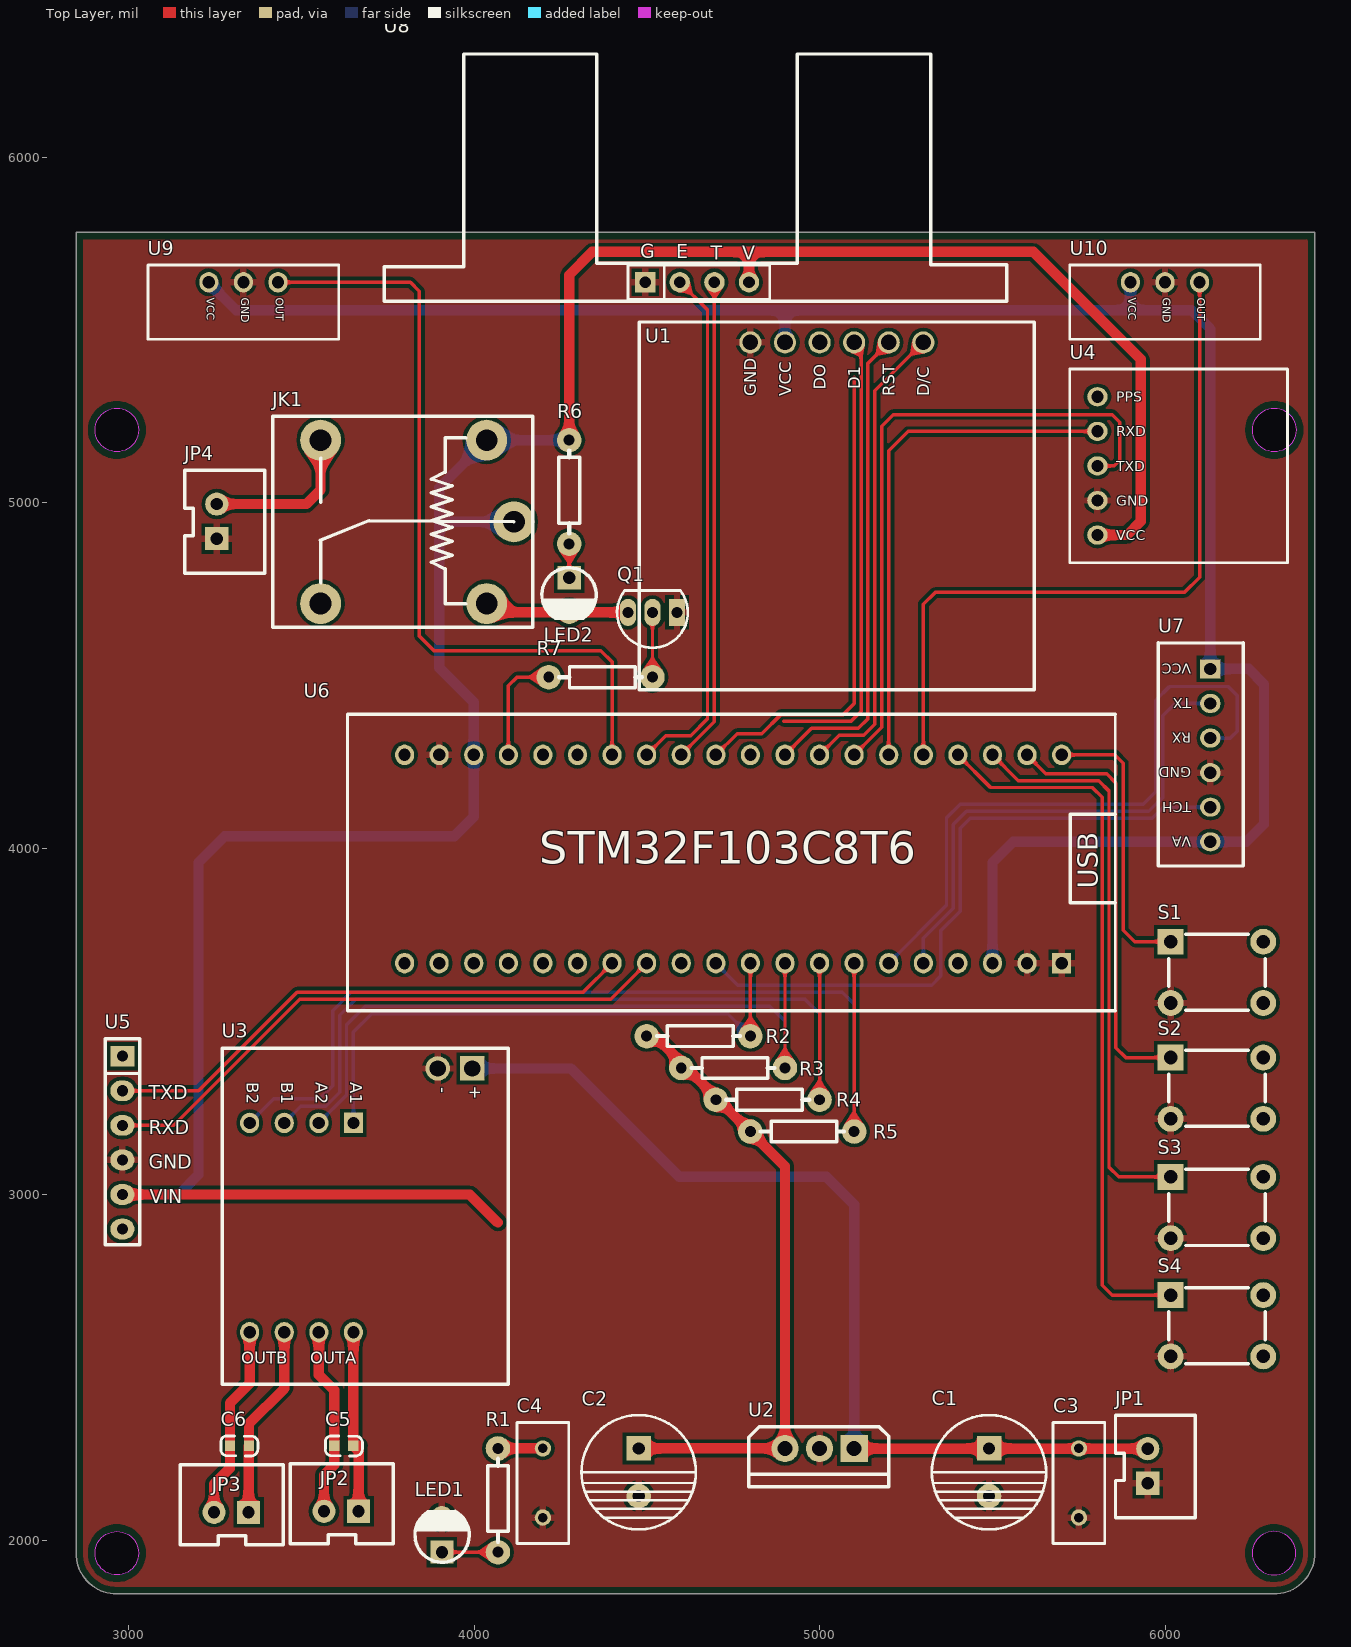
[diagram p0: Top Layer view]
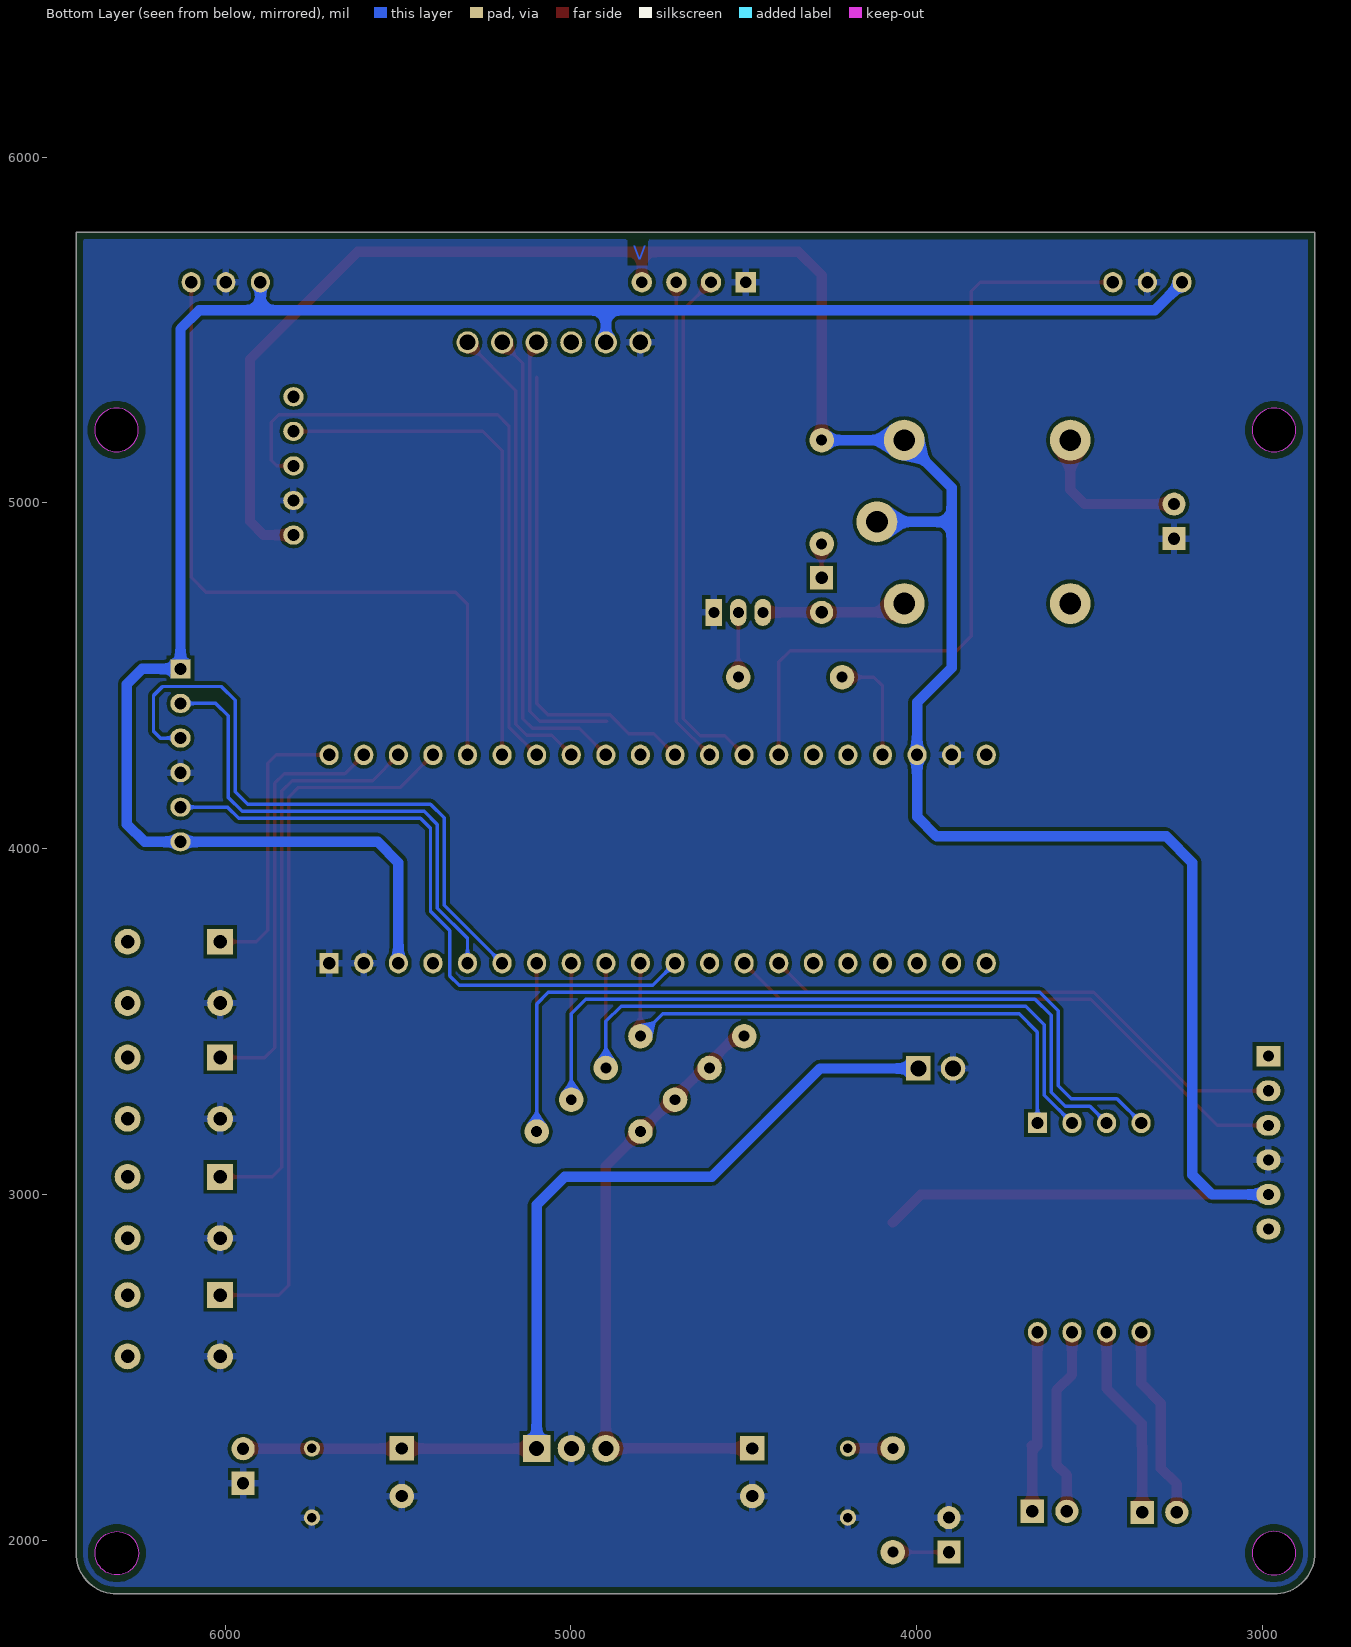
[diagram p1: Bottom Layer view, seen from below]
# Altium PCB MISC76356.PcbDoc
Units mil, origin at the board's own origin, x right, y up, seen from the top; angles counter-clockwise.
Board outline 3582.22 x 3937.22 mil, 2 copper layers (Top Layer, Bottom Layer); 35 components, 47 nets, 148 pads, 0 vias.
Unrouted connection lines stored in the file: 4.

## Layer stack, top to bottom (the 12.6 mil dielectric is the usual default, probably not edited)
Top Solder: solder mask 0.4, Solder Resist, Dk 3.5
Top Layer: signal copper 1.4
Dielectric 1: dielectric 12.6, FR-4, Dk 4.8
Bottom Layer: signal copper 1.4
Bottom Solder: solder mask 0.4, Solder Resist, Dk 3.5

## Board outline
2848.89,1963 ccw(c2967,1963) 2967,1844.89 6313,1844.89 ccw(c6313,1963) 6431.11,1963 6431.11,5782.11 2848.89,5781.99
cut-out: 6314,5148.04 cw(c6314,5211.03) 6251.01,5211.03 cw(c6314,5211.03) 6314,5274.02 cw(c6314,5211.03) 6376.99,5211.03 cw(c6314,5211.03)
cut-out: 2967,5148.04 cw(c2967,5211.03) 2904.01,5211.03 cw(c2967,5211.03) 2967,5274.02 cw(c2967,5211.03) 3029.99,5211.03 cw(c2967,5211.03)
cut-out: 6250.01,1963 ccw(c6313,1963) 6313,1900.01 ccw(c6313,1963) 6375.99,1963 ccw(c6313,1963) 6313,2025.99 ccw(c6313,1963)
cut-out: 2967,1900.01 cw(c2967,1963) 2904.01,1963 cw(c2967,1963) 2967,2025.99 cw(c2967,1963) 3029.99,1963 cw(c2967,1963)

## Design rules (kind name [scope] priority, off if disabled: settings)
BoardOutlineClearance [All] p1: gap=10 ignorepadtopadclearanceinfootprint=FALSE except(0: Arc-SplitContinuation Track-SplitContinuation SMDPad-SplitContinuation THPad-SplitContinuation Via-SplitContinuation Fill-SplitContinuation Poly-SplitContinuation Region-SplitContinuation Text-SplitContinuation; 20: Poly-OutlineEdge Poly-CavityEdge Poly-CutoutEdge Poly-SplitBarrior)
Clearance [All] p1: gap=10 ignorepadtopadclearanceinfootprint=FALSE except(0: Arc-Hole Track-Hole SMDPad-Hole THPad-Hole Via-Hole Fill-Hole Poly-Hole Region-Hole Text-Hole)
Height [All] p1: minheight=0 maxheight=4000 prefheight=500
PolygonConnect [All] p1: connectstyle=Relief reliefconductorwidth=20 reliefentries=4 polygonreliefangle="90 Angle" airgapwidth=10
RoutingVias [All] p1: holewidth=28 width=50 viastyle="Through Hole" minholewidth=28 minwidth=50 maxholewidth=28 maxwidth=50
SolderMaskExpansion [All] p1: expansion=4 istentingtop=FALSE
Width [All] p1: maxlimit=30 minlimit=10 preferedwidth=10
29 further rules are at their usual default settings.

## Components (designator, comment, footprint, x,y, rotation, side; value= is the part's Value field where it differs from the comment)
C1 "220uF/25V" DIP-EC3.5X8X11.5 5489,2265.8 r270 top value=100pF
C2 "220uF/25V" DIP-EC3.5X8X11.5 4476,2265.8 r270 top value=100pF
C3 "104" RAD-0.2 5749,2165.8 r90 top
C4 "104" RAD-0.2 4199,2165.8 r90 top
C5 "10uF" 0603C 3595.79,2274.35 r0 top
C6 "10uF" 0603C 3293.79,2274.35 r0 top
JK1 "SRD-05VDC-SL-C" SRD-C_B 4036.32,4709 r180 top
JP1 "2PIN" XH2.54-LI-2P 5948,2215 r90 top
JP2 "2PIN" XH2.54-LI-2P 3616,2084 r180 top
JP3 "2PIN" XH2.54-LI-2P 3298,2081 r180 top
JP4 "2PIN" XH2.54-LI-2P 3256,4946.62 r90 top
LED1 "LED" "LED 3MM-B" 3907,2015.8 r90 top
LED2 "LED" "LED 3MM-B" 4275,4733.41 r270 top
Q1 "9013" TO-92A 4586.73,4683.41 r180 top
R1 "1K" AXIAL0.3 4069,1965.8 r90 top
R2 "10K" AXIAL0.3 4499,3458 r0 top
R3 "10K" AXIAL0.3 4599,3366 r0 top
R4 "10K" AXIAL0.3 4699,3274 r0 top
R5 "10K" AXIAL0.3 4799,3182 r0 top
R6 "1K" AXIAL0.3 4275,4881.44 r90 top
R7 "10K" AXIAL0.3 4215.87,4496 r0 top
S1 "BUTTOM" DIP-6X6X5 6014.28,3731 r0 top
S2 "BUTTOM" DIP-6X6X5 6014.28,3396.17 r0 top
S3 "BUTTOM" DIP-6X6X5 6014.28,3051.17 r0 top
S4 "BUTTOM" DIP-6X6X5 6014.28,2709.17 r0 top
U1 "OLED-SPI" OLED-SPI 5049,5464 r0 top locked
U2 "LM7805" TO220A 4999,2265.8 r180 top
U3 "MX1508" 马达驱动芯片 3673.05,2983.12 r270 top
U4 "GPS module" GPS 5802.41,5107 r0 top
U5 "Header 6" "Pin HDR1X6/2.54mm-S" 2983,3400 r0 top
U6 "STM32F103" STM32FF103 4749,3970.18 r90 top
U7 "AS608" AS608 6129,4520 r180 top
U8 "HC-SR04" 超声波MODE 4645,5583 r0 top
U9 "IR pair" 火焰传感器 3333,5638 r270 top
U10 "IR pair" 火焰传感器 5998,5638 r270 top

## Footprints (in the part's own frame and the unit in brackets; to place one, negate y for a bottom-side part, rotate by r counter-clockwise, add the part's x,y. Pads: shape width x height; smd on the part's side, far side on the other; paste and mask are expansions set on the pad)
0603C [mil]
  rect 30x30 smd: 1(0.21,-0.35) 2(55.21,-1.35)
  silkscreen extent -26,-30 81,28, body extent -1,-15 62,17, height 12
AS608 [mm] "指纹模块"
  rect 1.5x1.4 hole 0.9: 1(0,0)
  oval 1.5x1.4 hole 0.9: 2(0,2.54) 3(0,5.08) 4(0,7.62) 5(0,10.16) 6(0,12.7)
  silkscreen extent -2.41,-1.91 3.81,14.48
AXIAL0.3 [mm]
  round 1.8 hole 0.8: 1(0,0) 2(7.62,0)
  silkscreen extent 0.76,-0.76 6.86,0.76, body extent -0.24,-1 7.86,1, height 1.25
DIP-6X6X5 [mm]
  rect 1.9x1.9 hole 1: 1(0,0)
  round 1.9 hole 1: 2(0,-4.5) 3(6.8,-4.5) 4(6.8,0)
  silkscreen extent -0.16,-5.04 6.96,0.54, body extent -0.8,-5.24 7.41,0.76, height 4.95
DIP-EC3.5X8X11.5 [mm]
  rect 1.8x1.8 hole 0.9: 1(0,0)
  round 1.8 hole 0.9: 2(3.5,0)
  silkscreen extent -2.45,-4.2 5.95,4.2, body extent -2.25,-4 5.75,4, height 11.53
GPS [mm]
  oval 1.5x1.4 hole 0.9: 1(0,5.08) 2(0,2.54) 3(0,0) 4(0,-2.54) 5(0,-5.08)
  silkscreen extent -2.03,-7.11 13.97,7.11, body extent -1.27,-6.35 1.27,6.35, height 8.5
"LED 3MM-B" [mm] "蓝色3mm直插LED"
  rect 1.7x1.7 hole 0.9: 1(-1.27,0)
  round 1.7 hole 0.9: 2(1.27,0)
  silkscreen extent -2.01,-2 1.72,1.98, body extent -1.95,-1.95 1.64,1.95, height 5.55
OLED-SPI [mil]
  round 64 hole 45: 1(-250,0) 2(-150,0) 3(-50,0) 4(50,0) 5(150,0) 6(250,0)
  silkscreen extent -571,-1004 571,59, body extent -300,-50 300,50, height 335
"Pin HDR1X6/2.54mm-S" [mil]
  rect 70x60 hole 32: 1(0,0)
  oval 70x60 hole 32: 2(0,-100) 3(0,-200) 4(0,-300) 5(0,-400) 6(0,-500)
  silkscreen extent -50,-545 50,50, body extent -50,-545 50,55, height 336
RAD-0.2 [mm] "Radial Cap, Thru-Hole; 2 Leads; 0.2 in Pin Spacing"
  round 1.2 hole 0.7: 1(-2.54,0) 2(2.54,0)
  silkscreen extent -4.45,-1.91 4.44,1.91
SRD-C_B [mm] "单刀双投"
  round 3 hole 1.6: 1(0,0) 2(0,-12) 3(-2,-6) 4(12.2,0) 5(12.2,-12)
  silkscreen extent -3.4,-13.75 15.7,1.75, body extent -3.33,-13.85 15.77,1.65, height 15.6
STM32FF103 [mm]
  rect 1.5x1.4 hole 0.9: 1(-7.65,-24.13)
  oval 1.5x1.4 hole 0.9: 2(-7.65,-21.59) 3(-7.65,-19.05) 4(-7.65,-16.51) 5(-7.65,-13.97) 6(-7.65,-11.43) 7(-7.65,-8.89) 8(-7.65,-6.35) 9(-7.65,-3.81) 10(-7.65,-1.27) 11(-7.65,1.27) 12(-7.65,3.81) 13(-7.65,6.35) 14(-7.65,8.89) 15(-7.65,11.43) 16(-7.65,13.97) 17(-7.65,16.51) 18(-7.65,19.05) 19(-7.65,21.59) 20(-7.65,24.13) 25(7.65,24.13) 26(7.65,21.59) 27(7.65,19.05) 28(7.65,16.51) 29(7.65,13.97) 30(7.65,11.43) 31(7.65,8.89) 32(7.65,6.35) 33(7.65,3.81) 34(7.65,1.27) 35(7.65,-1.27) 36(7.65,-3.81) 37(7.65,-6.35) 38(7.65,-8.89) 39(7.65,-11.43) 40(7.65,-13.97) 41(7.65,-16.51) 42(7.65,-19.05) 43(7.65,-21.59) 44(7.65,-24.13)
  silkscreen extent -11.15,-28.07 10.64,28.32, body extent -11.27,-26.99 11.23,31.65, height 20.7
TO220A [mm] "220，3脚晶体管"
  rect 2x2 hole 1.1: 1(-2.54,0)
  round 2 hole 1.1: 2(0,0) 3(2.54,0)
  silkscreen extent -5.08,-1.6 5.21,2.82, body extent -5.08,-1.45 5.22,2.98, height 18.5
TO-92A [mm]
  oval 1.2x2 hole 0.8: B(1.8,0) C(3.6,0)
  rect 1.2x2 hole 0.8: E(0,0)
  silkscreen extent -0.8,-1.6 4.4,2.6, body extent -0.5,-1.31 4.1,2.29, height 6.58
XH2.54-LI-2P [mm] "接插件，2P"
  rect 1.7x1.7 hole 0.9: 1(-1.27,0)
  round 1.7 hole 0.9: 2(1.27,0)
  silkscreen extent -3.81,-3.51 3.74,2.37, body extent -3.77,-3.3 3.77,2.4, height 7.05
火焰传感器 [mm]
  oval 1.5x1.4 hole 0.9: 1(0,-2.54) 2(0,0) 3(0,2.54)
  silkscreen extent -1.27,-7 4.19,7
超声波MODE [mm]
  rect 1.5x1.5 hole 0.85: 1(-3.81,1.397)
  round 1.5 hole 0.85: 2(-1.27,1.397) 3(1.27,1.397) 4(3.81,1.397)
  silkscreen extent -22.99,0 22.73,18.16, body extent -22.23,1.07 22.77,19.14, height 28.63
马达驱动芯片 [mm]
  rect 1.5x1.4 hole 0.9: 1(-5.687,-0.56)
  oval 1.5x1.4 hole 0.9: 2(-5.687,-3.1) 3(-5.686,-5.64) 4(-5.686,-8.18) 5(9.686,-8.18) 6(9.687,-5.64) 7(9.687,-3.1) 8(9.687,-0.56)
  rect 1.8x1.8 hole 1.2: 9(-9.687,8.18)
  round 1.8 hole 1.2: 10(-9.687,5.64)
  silkscreen extent -11.19,-10.18 13.51,10.82

## Part data
C1 C2: library part "Cap Pol2", "Polarized Capacitor (Axial)"
C3 C4 C5 C6: library part CAP, "non-polarized capacitor"
JK1: "5V single-group converter"
Q1: library part 2N3904, "NPN General Purpose Amplifier"
R1 R2 R3 R4 R5 R6 R7: library part RES, "resistor"
S1 S2 S3 S4: "push button"
U3: library part 马达驱动模块, "Motor driver module"
U4: library part GPS
U5: "Header, 6-Pin"
U7: library part 指纹模块
U8: library part 超声波MODE, "Ultrasonic module"
U9 U10: library part "Pin HDR1X3"

## Nets (pads, with @x,y where several pads share a name; then routed paths per layer and width w, separated by ;. In a path a pad name is that pad's centre, name@x,y a point inside that pad or via, vN(x,y) a via of type N, cw(c..) or ccw(c..) an arc to the next point about the centre after c; other vN are vias at no path point)
3V3: U1.2 U6.3 U6.25 U7.1 U7.6 U9.1 U10.1 | length 5810.3
  Bottom Layer w30: U9.1 3233,5636.03 3312.03,5557 4899,5557 ; U1.2 4899,5557 ; U6.3 5499,3960 5559,4020 U7.6 6233,4020 6284,4071 6284,4476 6240,4520 U7.1 6129,5503 6075,5557 5898,5557 ; U10.1 5898,5557 ; 4899,5557 5898,5557
5V: C2.1 C4.2 JK1.2 JK1.3 R1.2 R2.1 R3.1 R4.1 R5.1 R6.2 U2.3 U4.5 U5.5 U6.27 U8.4 | length 9670.6
  Top Layer w30: U5.5 3988,3000 4069,2919 ; R1.2 C4.2 ; R6.2 4275,5659 4342,5726 4795,5726 ; C2.1 U2.3 4899,3082 R5.1 4530.82,3450.18 4506.82,3450.18 R2.1 ; R3.1@4598.24,3365.24 R3.1 ; U8.4 4795,5726 ; U4.5 5888,4907 5928,4947 5928,5415 5617,5726 4795,5726
  Bottom Layer w30: U5.5 3146,3000 3203,3057 3203,3960 3279,4036 3943,4036 3999,4092 U6.27 3999,4423 3899,4523 3899,4945.22 ; JK1.3 3899,4945.22 ; R6.2 JK1.2 3899,5044.13 3899,4945.22
GND: C1.2 C2.2 C3.1 C4.1 JP1.1 JP4.1 LED1.2 Q1.E S1.2 S2.2 S3.2 S4.2 U1.1 U2.2 U3.10 U4.4 U5.4 U6.1 U6.2 U6.26 U7.4 U8.1 U9.2 U10.2
NetC5_1: C5.1 JP2.2 U3.7 | length 548.8
  Top Layer w30: U3.7 3551,2479 3596,2434 C5.1 3596,2219 3566,2189 JP2.2
NetC5_2: C5.2 JP2.1 U3.8 | length 541.4
  Top Layer w30: U3.8 C5.2 C5.2@3666,2258 ; JP2.1 C5.2@3666,2258 ; 3667,2273 3666,2274 C5.2@3666,2258
NetC6_1: C6.1 JP3.2 U3.5 | length 564.3
  Top Layer w30: JP3.2 3249,2082 3248,2083 3248,2163 3294,2209 C6.1 3294,2397 3351,2454 U3.5
NetC6_2: C6.2 JP3.1 U3.6 | length 563.4
  Top Layer w30: JP3.1 3348,2272 C6.2 3349,2337 3451,2439 U3.6
NetJK1_1: JK1.1 LED2.2 Q1.C | length 386.6
  Top Layer w30: JK1.1@4058.41,4683.41 LED2.2 Q1.C
NetJK1_5: JK1.5 JP4.2 | length 460.6
  Top Layer w30: JP4.2 3514.62,4996.62 3556,5038 JK1.5
NetLED1_1: LED1.1 R1.1 | length 162
  Top Layer w10: LED1.1 R1.1
NetLED2_1: LED2.1 R6.1 | length 98
  Top Layer w10: LED2.1 R6.1
NetQ1_B: Q1.B R7.2 | length 187.4
  Top Layer w10: R7.2 Q1.B
PA0: U6.16
PA1: U6.15
PA2: U5.2 U6.14 | length 1568.8
  Top Layer w10: U5.2 3203,3300 3488,3585 4315,3585 U6.14
PA3: U5.3 U6.13 | length 1710.3
  Top Layer w10: U5.3 3131.28,3200 3496.28,3565 4395,3565 U6.13
PA4: U6.12
PA5: U6.11 U7.5 | length 1887.2
  Bottom Layer w10: U6.11 4763,3605 5323,3605 5350,3632 5350,3763.43 5406,3819.43 5406,4059 5435,4088 5961,4088 5993,4120 U7.5
PA6: R2.2 U3.1 U6.10 | length 1670.9
  Top Layer w10: R2.2 U6.10
  Bottom Layer w10: U3.1 3651,3470 3704,3523 4734,3523 R2.2
PA7: R3.2 U3.2 U6.9 | length 2063.7
  Top Layer w10: R3.2 U6.9
  Bottom Layer w10: U3.2 3631,3287 3631,3491 3685,3545 4855,3545 4899,3501 R3.2
PA8: U6.40 U10.3 | length 2119.9
  Top Layer w10: U6.40 5299,4707 5333,4741 6054,4741 6098,4785 U10.3
PA9: U4.2 U6.39 | length 1506.2
  Top Layer w10: U6.39 5199,5151 5255,5207 U4.2
PA10: U4.3 U6.38 | length 1875.8
  Top Layer w10: U6.38 5179,4351.36 5179,5222 5212,5255 5845,5255 5867,5233 5867,5123 5851,5107 U4.3
PA11: U1.6 U6.37 | length 1358.9
  Top Layer w10: U6.37 5055.64,4328 5127.35,4328 5159,4359.65 5159,5324 U1.6
PA12: U1.5 U6.36 | length 1396.2
  Top Layer w10: U6.36 4975.64,4348 5111,4348 5139,4376 5139,5404 U1.5
PA15: U1.4 U6.35 | length 1298.4
  Top Layer w10: 4895.64,4368 5090,4368 5119,4397 U1.4@5119,5460
PB0: R4.2 U3.3 U6.8 | length 2488.1
  Top Layer w10: R4.2 U6.8
  Bottom Layer w10: U3.3 3499,3255 3570.72,3255 3611,3295.28 3611,3518 3658,3565 4957,3565 4999,3523 R4.2
PB1: R5.2 U3.4 U6.7 | length 2901.8
  Top Layer w10: R5.2 U6.7
  Bottom Layer w10: U3.4 3421,3277 3553,3277 3591,3315 3591,3532 3644,3585 5065,3585 5099,3551 R5.2
PB3: U1.3 U6.34 | length 1405.6
  Top Layer w10: U6.34 4760.64,4333 4832.35,4333 4887.35,4388 5067,4388 5099,4420 5099,5364
PB4: U6.33 U8.3 | length 1406.4
  Top Layer w10: U6.33 4695,4367.36 U8.3
PB5: U6.32 U8.2 | length 1514.7
  Top Layer w10: U6.32 4554.64,4327 4626.35,4327 4675,4375.65 4675,5558 U8.2
PB6: U6.31 U9.3 | length 2273.5
  Top Layer w10: U9.3 3816,5638 3842,5612 3842,4615 3884,4573 4366,4573 4399,4540 U6.31
PB7: U6.30
PB8: U6.29
PB9: R7.1 U6.28 | length 326.9
  Top Layer w10: U6.28 4099,4471 4124,4496 R7.1
PB10: U6.6 U7.3 | length 1842.3
  Bottom Layer w10: U6.6 5366,3836 5366,4089 5406,4129 5935,4129 5971,4165 5971,4429 6011,4469 6181,4469 6207,4443 6207,4340 6187,4320 U7.3
PB11: U6.5 U7.2 | length 1463.3
  Bottom Layer w10: U6.5 5299,3740.72 5386,3827.72 5386,4070 5424,4108 5951,4108 5991,4148 5991,4384 6027,4420 U7.2
PB12: S1.1 S1.4 U6.44 | length 822
  Top Layer w10: U6.44 5852.64,4271.36 5877,4247 5877,3764 5910,3731 S1.1
PB13: S2.1 S2.4 U6.43 | length 1225.9
  Top Layer w10: U6.43 5653.36,4217 5829,4217 5856,4190 5856,3425 5884.83,3396.17 S2.1
PB14: S3.1 S3.4 U6.42 | length 1658
  Top Layer w10: U6.42 5573.36,4197 5806,4197 5836,4167 5836,3079 5863.83,3051.17 S3.1
PB15: S4.1 S4.4 U6.41 | length 2088.9
  Top Layer w10: U6.41 5493.36,4177 5788,4177 5816,4149 5816,2738 5844.83,2709.17 S4.1
PC13: U6.19
PC14: U6.18
PC15: U6.17
R: U6.4
VB: U6.20
VBAT: C1.1 C3.2 JP1.2 U2.1 U3.9 | length 2821.9
  Top Layer w30: U3.9 U3.9@3995.85,3365.24 ; U2.1 5099.4,2265.4 5947.6,2265.4 JP1.2
  Bottom Layer w30: U3.9 4279.52,3364.48 4593,3051 5018,3051 5099,2970 U2.1
pads on no net: JK1.4 S1.3 S2.3 S3.3 S4.3 U4.1 U5.1 U5.6

## Polygon pours and split planes (outlines as drawn)
GND on Bottom Layer "NONET_L-01_P-001" (solid, pour order 1): 2786,5960 2786,1851 2939,1698 6440,1698 6440,5837 6249,6028
GND on Top Layer "NONET_L-01_P-001" (solid, pour order 0): 2743,6022 2700,5979 2700,1729 6402,1729 6673,2000 6673,5862

## Silkscreen, mask and mechanical layers (free items; w line width, h text height)
Top Overlay:
  text "TXD" at 3058.67,3275.01 h40
  text "RXD" at 3058.67,3175.01 h40
  text "GND" at 3058.67,3075.01 h40
  text "VIN" at 3062,2975.01 h40
Mechanical 1:
  circle w10: c6314,5211.03 r62.99
  circle w10: c2967,5211.03 r62.99
  circle w10: c6313,1963 r62.99
  circle w10: c2967,1963 r62.99
  lines w10: 2848.89,1963 ccw(c2967,1963) 2967,1844.89 6313,1844.89 ccw(c6313,1963) 6431.11,1963 6431.11,5782.11 2848.89,5781.99 2848.89,1963